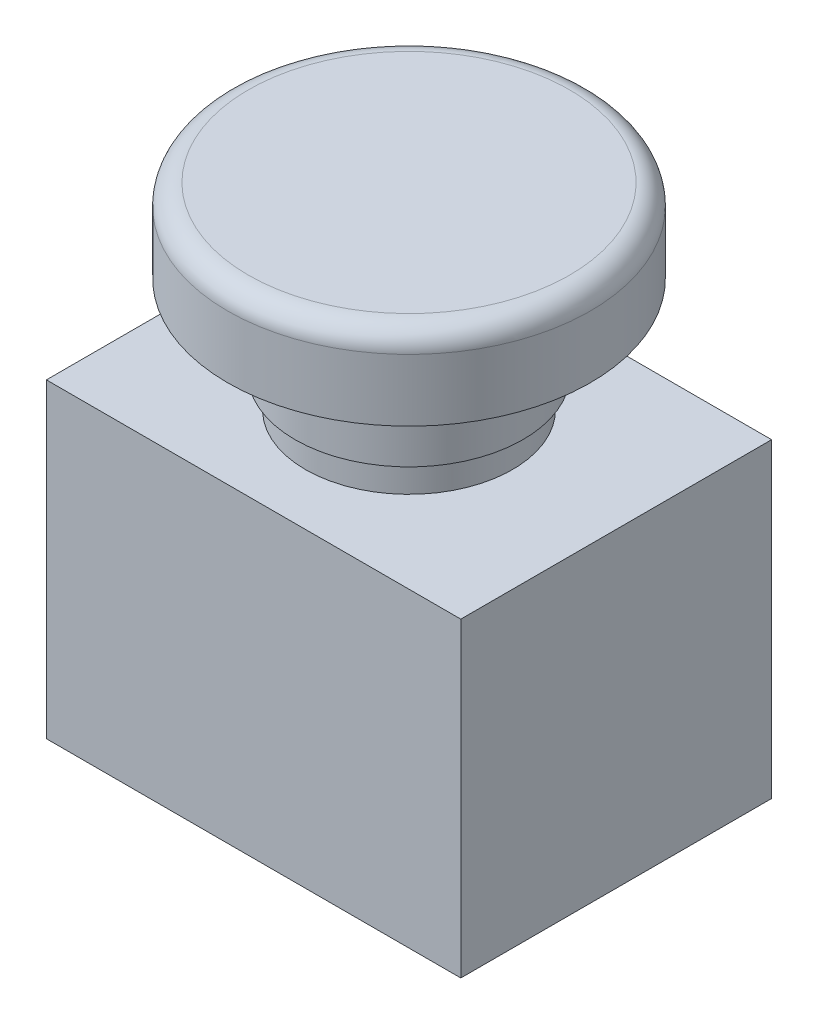
SolidWorks part; units mm, degrees
ref_plane "Front Plane" through (0, 0, 0) normal (0, 0, 1) x (1, 0, 0)
ref_plane "Top Plane" through (0, 0, 0) normal (0, 1, 0) x (1, 0, 0)
ref_plane "Right Plane" through (0, 0, 0) normal (1, 0, 0) x (0, 0, -1)
sketch "Sketch1" plane through (0, 0, 0) normal (0, 1, 0) x (1, 0, 0)
  line L0 (20, 15) -> (-20, -15) construction
  line L1 (-20, 15) -> (20, 15)
  line L2 (-20, 15) -> (-20, -15)
  line L3 (-20, -15) -> (20, -15)
  line L4 (20, 15) -> (20, -15)
  dimension "D1" = 40
  dimension "D2" = 30
extrude "Extrude1" add sketch "Sketch1" along normal mid plane 30
other "Double-side Block<1>"
sketch "Sketch2" plane through (0, 15, 0) normal (0, 1, 0) x (1, 0, 0)
  circle A0 centre (0, 0) radius 11
  dimension "D1" = 22
extrude "Extrude2" add sketch "Sketch2" along normal blind 10
sketch "Sketch3" plane through (0, 25, 0) normal (0, 1, 0) x (1, 0, 0)
  circle A0 centre (0, 0) radius 10
  dimension "D1" = 20
extrude "Extrude3" add sketch "Sketch3" along normal blind 1
sketch "Sketch4" plane through (0, 26, 0) normal (0, 1, 0) x (1, 0, 0)
  circle A0 centre (0, 0) radius 17.5
  dimension "D1" = 35
extrude "Extrude4" add sketch "Sketch4" along normal blind 8
fillet "Fillet1" radius 2 1 edges at (0, 34, 17.5)
ref_plane "Plane1" through (0, 18, 0) normal (0, 1, 0) x (-1, 0, 0)
sketch "Sketch5" plane through (0, 18, 0) normal (0, 1, 0) x (-1, 0, 0)
  circle A0 centre (0, 0) radius 10
  dimension "D1" = 20
extrude "Cut-Extrude1" cut sketch "Sketch5" against normal blind 3 flip side to cut
